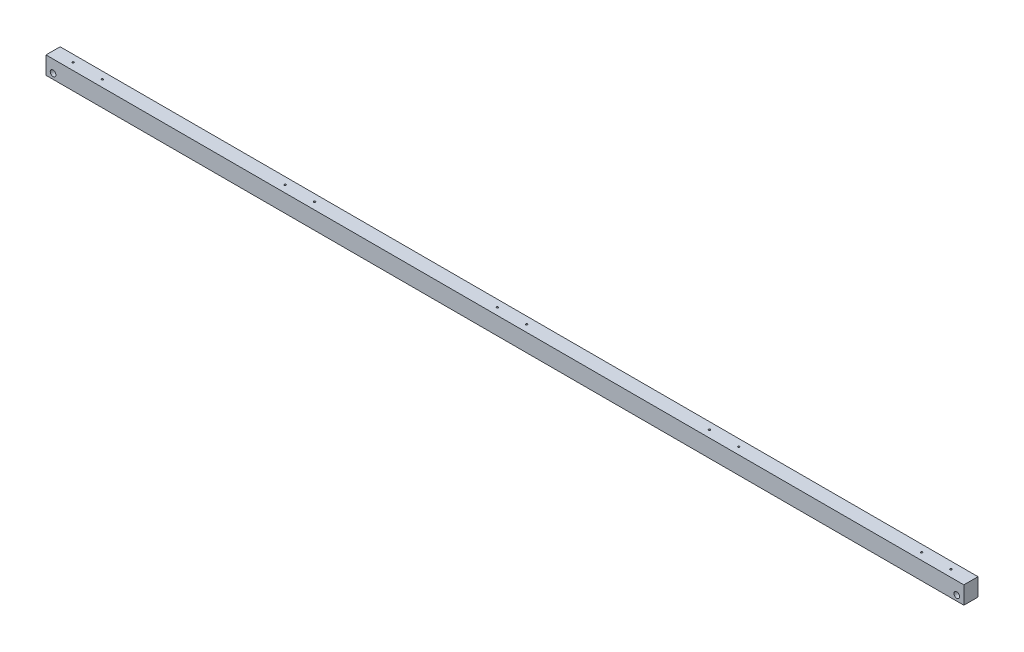
SolidWorks part; units mm, degrees
ref_plane "Front Plane" through (0, 0, 0) normal (0, 0, 1) x (1, 0, 0)
ref_plane "Top Plane" through (0, 0, 0) normal (0, 1, 0) x (1, 0, 0)
ref_plane "Right Plane" through (0, 0, 0) normal (1, 0, 0) x (0, 0, -1)
sketch "Sketch1" plane through (0, 0, 0) normal (0, 1, 0) x (1, 0, 0)
  line L1 (-1298, -20) -> (1298, -20)
  line L2 (-1298, -20) -> (-1298, 20)
  line L3 (-1298, 20) -> (1298, 20)
  line L4 (1298, -20) -> (1298, 20)
  line L5 (-1298, -20) -> (1298, 20) construction
  line L6 (-1298, 20) -> (1298, -20) construction
  point P0 (0, 0)
  dimension "D1" = 2596
  dimension "D2" = 40
extrude "Boss-Extrude1" add sketch "Sketch1" along normal blind 50
sketch "Sketch2" plane through (0, 0, 0) normal (0, -1, 0) x (1, 0, 0)
  line L0 (1298, 20) -> (1298, -20) construction
  line L1 (1298, -20) -> (-1298, -20) construction
  line L2 (1298, 0) -> (-1298, 0) construction
  line L3 (-1298, -20) -> (-1298, 20) construction
  line L4 (0, 0) -> (0, 93.7698) construction
  circle A0 centre (1241.5, 0) radius 2.5
  circle A1 centre (1158.5, 0) radius 2.5
  circle A2 centre (641.5, 0) radius 2.5
  circle A3 centre (558.5, 0) radius 2.5
  circle A4 centre (41.5, 0) radius 2.5
  circle A5 centre (-41.5, 0) radius 2.5
  circle A6 centre (-558.5, 0) radius 2.5
  circle A7 centre (-641.5, 0) radius 2.5
  circle A8 centre (-1158.5, 0) radius 2.5
  circle A9 centre (-1241.5, 0) radius 2.5
  dimension "D1" = 5
  dimension "D5" = 5
  dimension "D6" = 5
  dimension "D9" = 5
  dimension "D10" = 5
  dimension "D2" = 56.5
  dimension "D3" = 20
  dimension "D4" = 83
  dimension "D7" = 517
  dimension "D8" = 83
  dimension "D11" = 517
extrude "Cut-Extrude1" cut sketch "Sketch2" against normal blind 50
sketch "Sketch3" plane through (0, 0, -20) normal (0, 0, -1) x (-1, 0, 0)
  line L0 (-1298, 50) -> (-1298, 0) construction
  line L1 (-1298, 50) -> (1298, 50) construction
  line L2 (0, 0) -> (0, 177.2599) construction
  circle A0 centre (-1278, 15) radius 8
  circle A1 centre (1278, 15) radius 8
  dimension "D1" = 16
  dimension "D2" = 20
  dimension "D3" = 35
extrude "Cut-Extrude2" cut sketch "Sketch3" against normal blind 50
